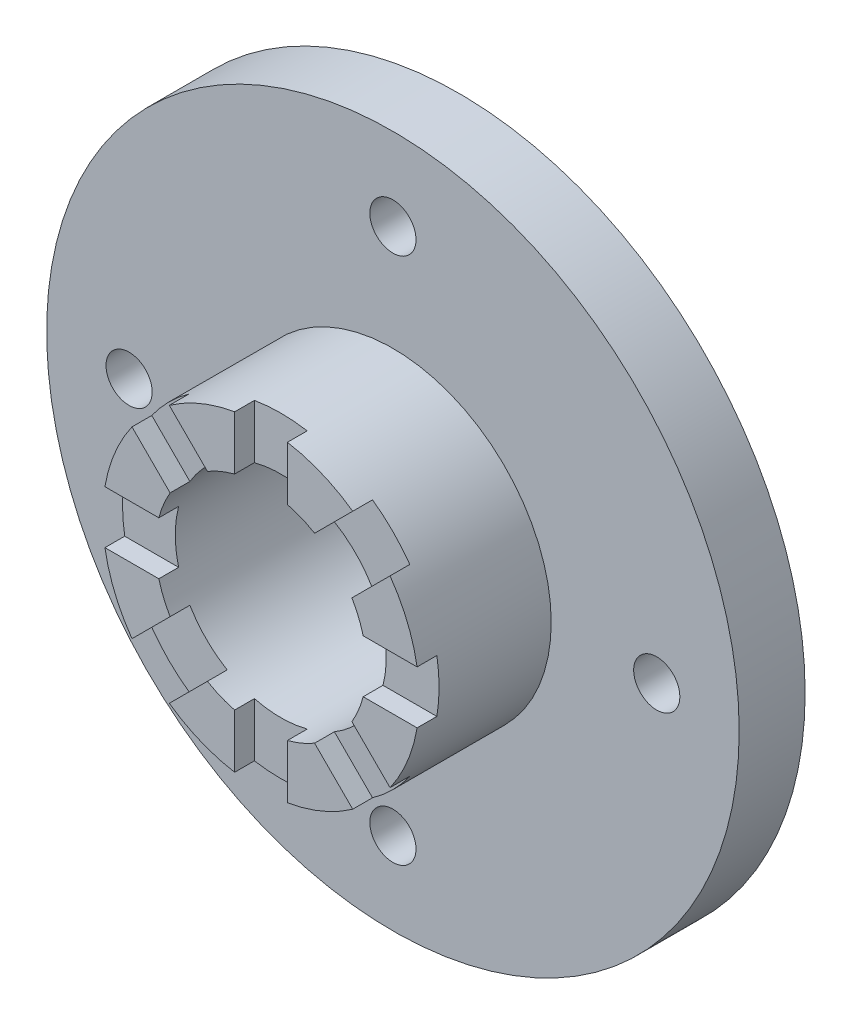
SolidWorks part; units mm, degrees
ref_plane "前视基准面" through (0, 0, 0) normal (0, 0, 1) x (1, 0, 0)
ref_plane "上视基准面" through (0, 0, 0) normal (0, 1, 0) x (1, 0, 0)
ref_plane "右视基准面" through (0, 0, 0) normal (1, 0, 0) x (0, 0, -1)
sketch "草图1" plane through (0, 0, 0) normal (0, 0, 1) x (1, 0, 0)
  circle A0 centre (0, 0) radius 52.5
  circle A1 centre (0, 0) radius 24
  circle A2 centre (0, 0) radius 16
  circle A3 centre (0, 0) radius 40 construction
  circle A4 centre (0, 40) radius 3.5
  circle A5 centre (40, 0) radius 3.5
  circle A6 centre (0, -40) radius 3.5
  circle A7 centre (-40, 0) radius 3.5
  dimension "D1" = 105
  dimension "D2" = 48
  dimension "D3" = 32
  dimension "D4" = 80
  dimension "D5" = 7
  dimension "D6" = 4
extrude "凸台-拉伸1" add sketch "草图1" along normal blind 10 contours A0 A1 | A1 A2
cosmetic thread "装饰螺纹线1" parameters "D2"=36
sketch "草图2" plane through (0, 0, 10) normal (0, 0, 1) x (1, 0, 0)
  circle A0 centre (0, 0) radius 16 construction
  circle A1 centre (0, 0) radius 16
  circle A2 centre (0, 0) radius 24 construction
  circle A3 centre (0, 0) radius 24
extrude "凸台-拉伸2" add sketch "草图2" along normal blind 20
sketch "草图3" plane through (0, 0, 30) normal (0, 0, 1) x (1, 0, 0)
  line L0 (0, 24) -> (0, 16) construction
  line L1 (-4, 23.6643) -> (-4, 15.4919)
  line L2 (4, 23.6643) -> (4, 15.4919)
  line L3 (13.9048, 19.5616) -> (8.126, 13.7829)
  line L4 (19.5616, 13.9048) -> (13.7829, 8.126)
  line L5 (23.6643, 4) -> (15.4919, 4)
  line L6 (23.6643, -4) -> (15.4919, -4)
  line L7 (19.5616, -13.9048) -> (13.7829, -8.126)
  line L8 (13.9048, -19.5616) -> (8.126, -13.7829)
  line L9 (4, -23.6643) -> (4, -15.4919)
  line L10 (-4, -23.6643) -> (-4, -15.4919)
  line L11 (-13.9048, -19.5616) -> (-8.126, -13.7829)
  line L12 (-19.5616, -13.9048) -> (-13.7829, -8.126)
  line L13 (-23.6643, -4) -> (-15.4919, -4)
  line L14 (-23.6643, 4) -> (-15.4919, 4)
  line L15 (-19.5616, 13.9048) -> (-13.7829, 8.126)
  line L16 (-13.9048, 19.5616) -> (-8.126, 13.7829)
  circle A0 centre (0, 0) radius 24 construction
  arc A1 (4, 23.6643) -> (-4, 23.6643) centre (0, 0) ccw
  circle A2 centre (0, 0) radius 16 construction
  arc A3 (4, 15.4919) -> (-4, 15.4919) centre (0, 0) ccw
  arc A4 (19.5616, 13.9048) -> (13.9048, 19.5616) centre (0, 0) ccw
  arc A5 (13.7829, 8.126) -> (8.126, 13.7829) centre (0, 0) ccw
  arc A6 (23.6643, -4) -> (23.6643, 4) centre (0, 0) ccw
  arc A7 (15.4919, -4) -> (15.4919, 4) centre (0, 0) ccw
  arc A8 (8.126, -13.7829) -> (13.7829, -8.126) centre (0, 0) ccw
  arc A9 (13.9048, -19.5616) -> (19.5616, -13.9048) centre (0, 0) ccw
  arc A10 (-4, -23.6643) -> (4, -23.6643) centre (0, 0) ccw
  arc A11 (-4, -15.4919) -> (4, -15.4919) centre (0, 0) ccw
  arc A12 (-19.5616, -13.9048) -> (-13.9048, -19.5616) centre (0, 0) ccw
  arc A13 (-13.7829, -8.126) -> (-8.126, -13.7829) centre (0, 0) ccw
  arc A14 (-23.6643, 4) -> (-23.6643, -4) centre (0, 0) ccw
  arc A15 (-15.4919, 4) -> (-15.4919, -4) centre (0, 0) ccw
  arc A16 (-13.9048, 19.5616) -> (-19.5616, 13.9048) centre (0, 0) ccw
  arc A17 (-8.126, 13.7829) -> (-13.7829, 8.126) centre (0, 0) ccw
  dimension "D1" = 4
  dimension "D2" = 8
extrude "切除-拉伸2" cut sketch "草图3" against normal blind 3
